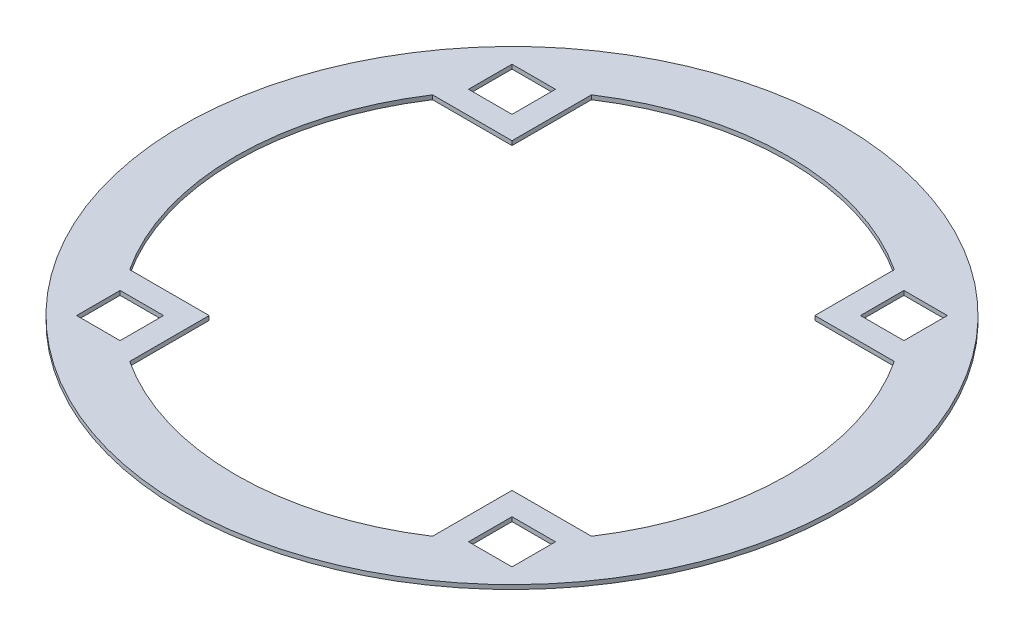
from build123d import *

# Parameters (mm, degrees)
SKETCH_1_R      = 925
SKETCH_1_W      = 122
SKETCH_1_H      = 122
EXTRUDE_1_DEPTH = 12


with BuildPart() as part:
    # 草图1 → 凸台-拉伸1 (new body)
    with BuildSketch(Plane(origin=(0, 0, 0), x_dir=(1, 0, 0), z_dir=(0, 1, 0))):
        with Locations(Location((0, 0, 0), (0, 0, 270))):
            Circle(SKETCH_1_R)
        with BuildLine():
            Line((-648.074069841, 425), (-425, 425))
            Line((-425, 425), (-425, 648.074069841))
            ThreePointArc((-425, 648.074069841), (0, 775), (425, 648.074069841))
            Line((425, 648.074069841), (425, 425))
            Line((425, 425), (648.074069841, 425))
            ThreePointArc((648.074069841, 425), (775, 0), (648.074069841, -425))
            Line((648.074069841, -425), (425, -425))
            Line((425, -425), (425, -648.074069841))
            ThreePointArc((425, -648.074069841), (0, -775), (-425, -648.074069841))
            Line((-425, -648.074069841), (-425, -425))
            Line((-425, -425), (-648.074069841, -425))
            ThreePointArc((-648.074069841, -425), (-775, 0), (-648.074069841, 425))
        make_face(mode=Mode.SUBTRACT)
        with Locations((-550, 550)):
            Rectangle(SKETCH_1_W, SKETCH_1_H, mode=Mode.SUBTRACT)
        with Locations((-550, -550)):
            Rectangle(SKETCH_1_W, SKETCH_1_H, mode=Mode.SUBTRACT)
        with Locations((550, -550)):
            Rectangle(SKETCH_1_W, SKETCH_1_H, mode=Mode.SUBTRACT)
        with Locations((550, 550)):
            Rectangle(SKETCH_1_W, SKETCH_1_H, mode=Mode.SUBTRACT)
    extrude(amount=EXTRUDE_1_DEPTH)


solid = part.part
